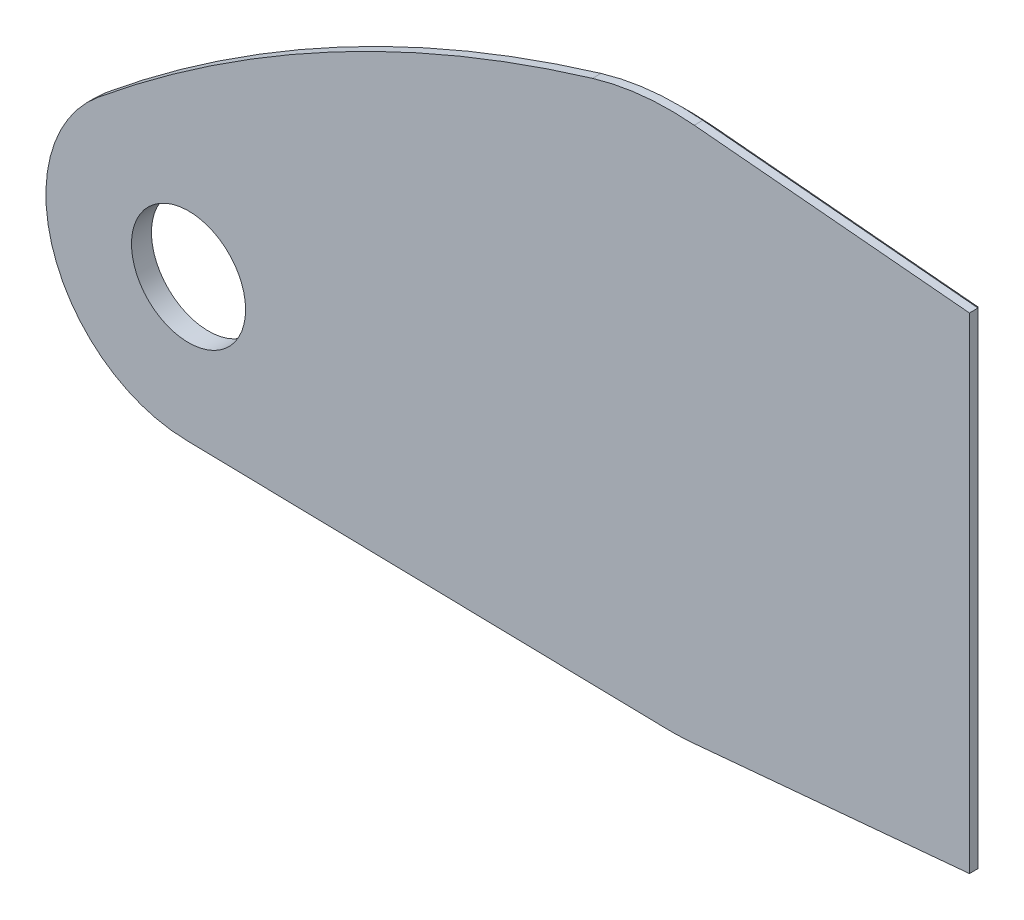
from build123d import *

# Parameters (mm, degrees)
SKETCH1_R           = 40
BOSS_EXTRUDE1_DEPTH = 14
CHAMFER1_SIZE       = 8


with BuildPart() as part:
    # Sketch1 → Boss-Extrude1 (new body)
    with BuildSketch(Plane.XY):
        with BuildLine():
            Line((210, 170.2), (17.052877352, 187.727060846))
            ThreePointArc((17.052877352, 187.727060846), (-18.959205139, 187.54412425), (-54.27928922, 180.515951544))
            ThreePointArc((-54.27928922, 180.515951544), (-236.788094268, 105.291584642), (-400.963833305, -4.319071808))
            ThreePointArc((-400.963833305, -4.319071808), (-431.989523554, -114.33728667), (-339.549522969, -181.578995072))
            Line((-339.549522969, -181.578995072), (-3.863350797, -188.460405711))
            ThreePointArc((-3.863350797, -188.460405711), (6.604949005, -188.384247347), (17.052877352, -187.727060846))
            Line((17.052877352, -187.727060846), (210, -170.2))
            Line((210, -170.2), (210, 170.2))
        make_face()
        with Locations((-337.5, -81.6)):
            Circle(SKETCH1_R, mode=Mode.SUBTRACT)
    extrude(amount=BOSS_EXTRUDE1_DEPTH)

    # Chamfer1
    chamfer1_edges = [part.edges().sort_by_distance(p)[0] for p in [
        (-171.706436883, -185.019700391, 0),
        (-431.989523554, -114.33728667, 0),
        (-236.788094268, 105.291584642, 0),
        (-18.959205139, 187.54412425, 0),
        (113.526438676, 178.963530423, 0),
        (210, 0, 0),
        (113.526438676, -178.963530423, 0),
        (6.604949005, -188.384247347, 0),
    ]]
    chamfer(chamfer1_edges, length=CHAMFER1_SIZE)


solid = part.part
